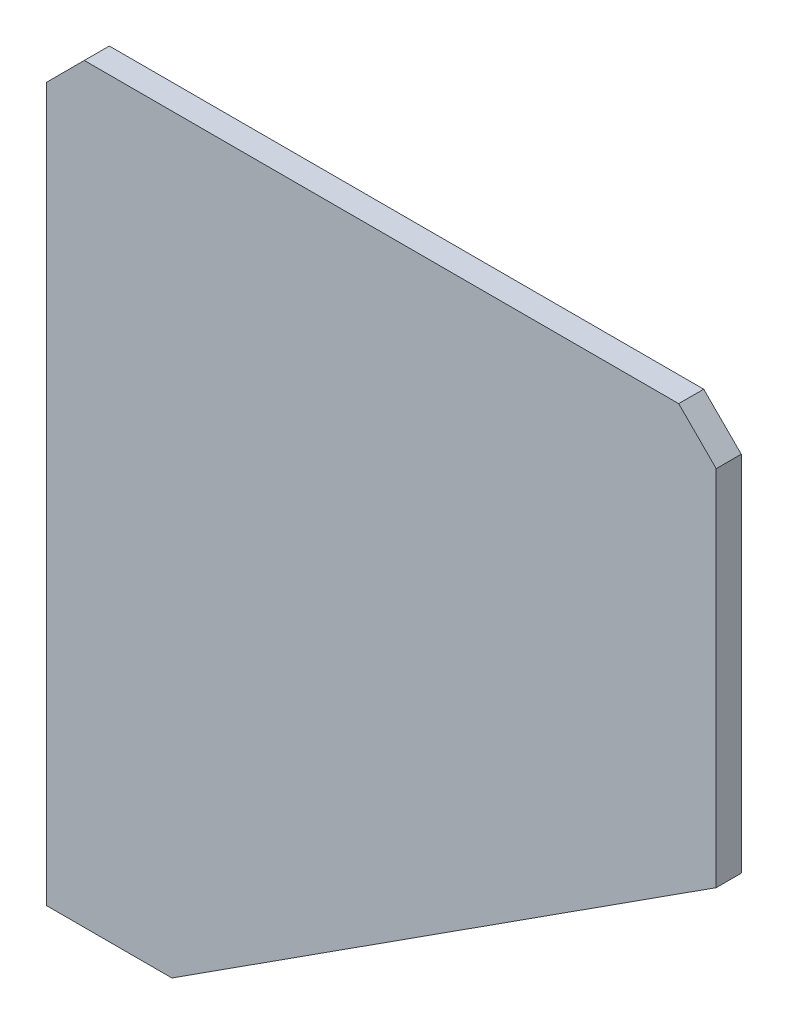
from build123d import *

# Parameters (mm, degrees)
EXTRUDE_1_DEPTH = 2
CHAMFER_1_SIZE  = 3


with BuildPart() as part:
    # 草图1 → 凸台-拉伸1 (new body)
    with BuildSketch(Plane.XY):
        Polygon((0, 0), (53.5, 0), (53.5, -32), (10, -60), (0, -60), align=None)
    extrude(amount=EXTRUDE_1_DEPTH)

    # 倒角1
    chamfer_1_edges = [part.edges().sort_by_distance(p)[0] for p in [
        (0, 0, 1),
        (53.5, 0, 1),
    ]]
    chamfer(chamfer_1_edges, length=CHAMFER_1_SIZE)


solid = part.part
